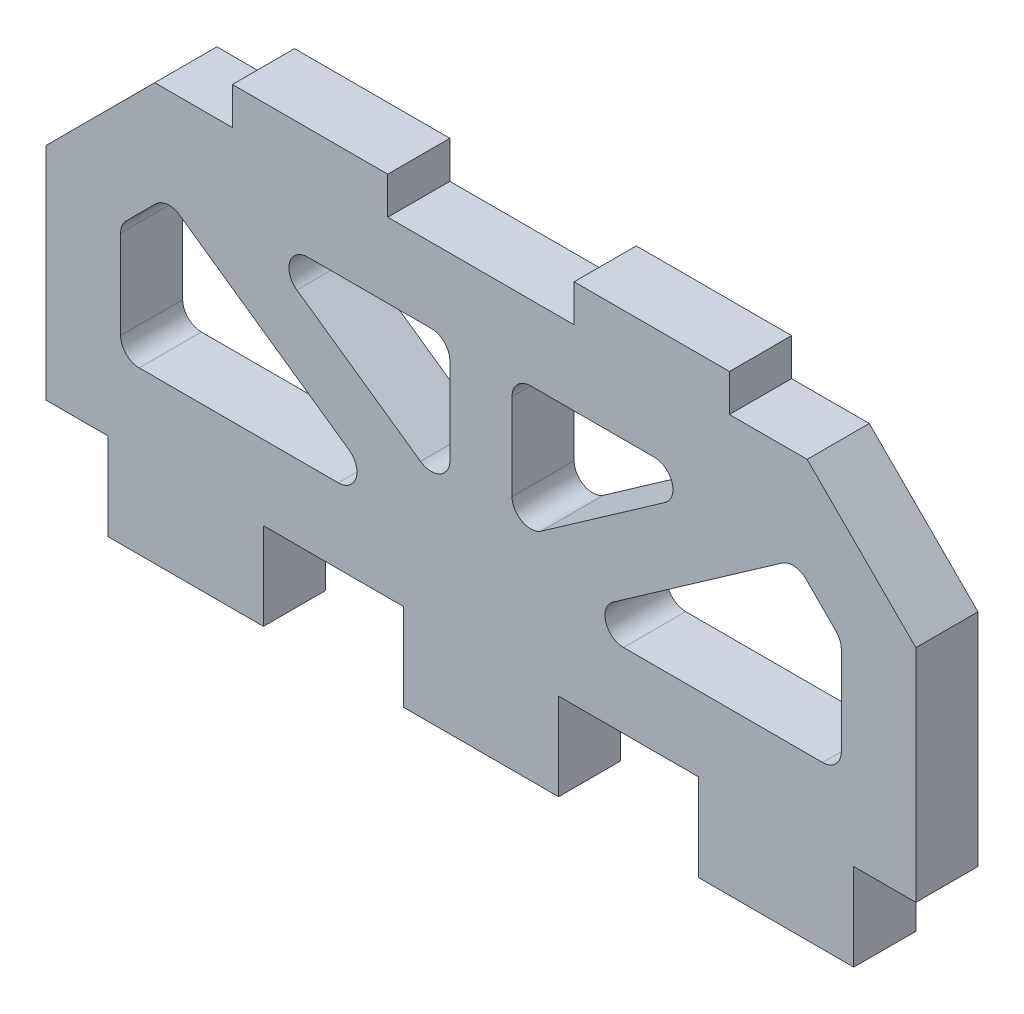
from build123d import *

# Parameters (mm, degrees)
EXTRUDE_1_DEPTH = 5
FILLET_3_R      = 1.5
FILLET_4_R      = 1.5
FILLET_5_R      = 1.5


with BuildPart() as part:
    # 草图1 → 凸台-拉伸1 (new body)
    with BuildSketch(Plane.XY):
        Polygon((7.785235828, 15.309450129), (-7.214764172, 15.309450129), (-7.214764172, 18.309450129), (-19.714764172, 18.309450129), (-19.714764172, 15.309450129), (-25.964764172, 15.309450129), (-34.714764172, 6.559450129), (-34.714764172, -11.190549871), (-29.714764172, -11.190549871), (-29.714764172, -18.207876603), (-17.214764172, -18.207876603), (-17.214764172, -11.190549871), (-5.964764172, -11.190549871), (-5.964764172, -18.207876603), (6.535235828, -18.207876603), (6.535235828, -11.190549871), (17.785235828, -11.190549871), (17.785235828, -18.207876603), (30.285235828, -18.207876603), (30.285235828, -11.190549871), (35.285235828, -11.190549871), (35.285235828, 6.559450129), (26.535235828, 15.309450129), (20.285235828, 15.309450129), (20.285235828, 18.309450129), (7.785235828, 18.309450129), align=None)
        Polygon((-24.987626131, 7.801306796), (-28.714764172, 4.074168755), (-28.714764172, -5.190549871), (-6.433331929, -5.190549871), align=None, mode=Mode.SUBTRACT)
        Polygon((-18.424244048, 9.309450129), (-2.214764172, 9.309450129), (-2.214764172, -2.040549871), align=None, mode=Mode.SUBTRACT)
        Polygon((2.785235828, -2.040549871), (18.994715705, 9.309450129), (2.785235828, 9.309450129), align=None, mode=Mode.SUBTRACT)
        Polygon((7.003803585, -5.190549871), (25.558097787, 7.801306796), (29.285235828, 4.074168755), (29.285235828, -5.190549871), align=None, mode=Mode.SUBTRACT)
    extrude(amount=EXTRUDE_1_DEPTH)

    # 圆角3
    fillet_3_edges = [part.edges().sort_by_distance(p)[0] for p in [
        (-24.987626131, 7.801306796, 2.5),
    ]]
    fillet(fillet_3_edges, radius=FILLET_3_R)

    # 圆角4
    fillet_4_edges = [part.edges().sort_by_distance(p)[0] for p in [
        (-6.433331929, -5.190549871, 2.5),
        (-28.714764172, 4.074168755, 2.5),
        (-28.714764172, -5.190549871, 2.5),
    ]]
    fillet(fillet_4_edges, radius=FILLET_4_R)

    # 圆角5
    fillet_5_edges = [part.edges().sort_by_distance(p)[0] for p in [
        (29.285235828, -5.190549871, 2.5),
        (29.285235828, 4.074168755, 2.5),
        (25.558097787, 7.801306796, 2.5),
        (-18.424244048, 9.309450129, 2.5),
        (-2.214764172, -2.040549871, 2.5),
        (-2.214764172, 9.309450129, 2.5),
        (2.785235828, 9.309450129, 2.5),
        (2.785235828, -2.040549871, 2.5),
        (18.994715705, 9.309450129, 2.5),
        (7.003803585, -5.190549871, 2.5),
    ]]
    fillet(fillet_5_edges, radius=FILLET_5_R)


solid = part.part
